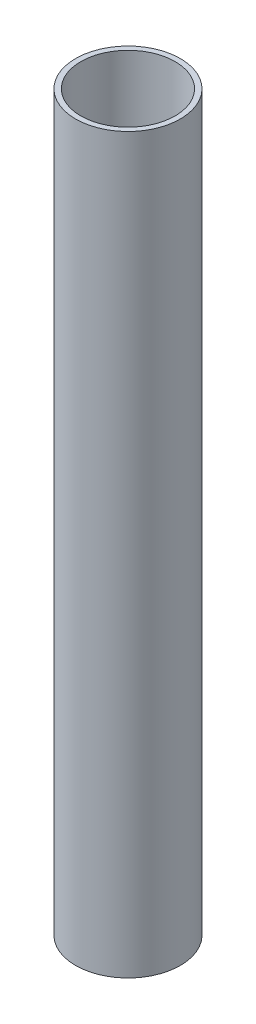
SolidWorks part; units mm, degrees
material "Thornel Mat VMA"
ref_plane "前视基准面" through (0, 0, 0) normal (0, 0, 1) x (1, 0, 0)
ref_plane "上视基准面" through (0, 0, 0) normal (0, 1, 0) x (1, 0, 0)
ref_plane "右视基准面" through (0, 0, 0) normal (1, 0, 0) x (0, 0, -1)
other "Configuration Table"
sketch "草图1" plane through (0, 0, 0) normal (0, 1, 0) x (1, 0, 0)
  circle A0 centre (0, 0) radius 9
  circle A1 centre (0, 0) radius 10
  dimension "D1" = 18
  dimension "D2" = 20
extrude "凸台-拉伸1" add sketch "草图1" along normal blind 140
